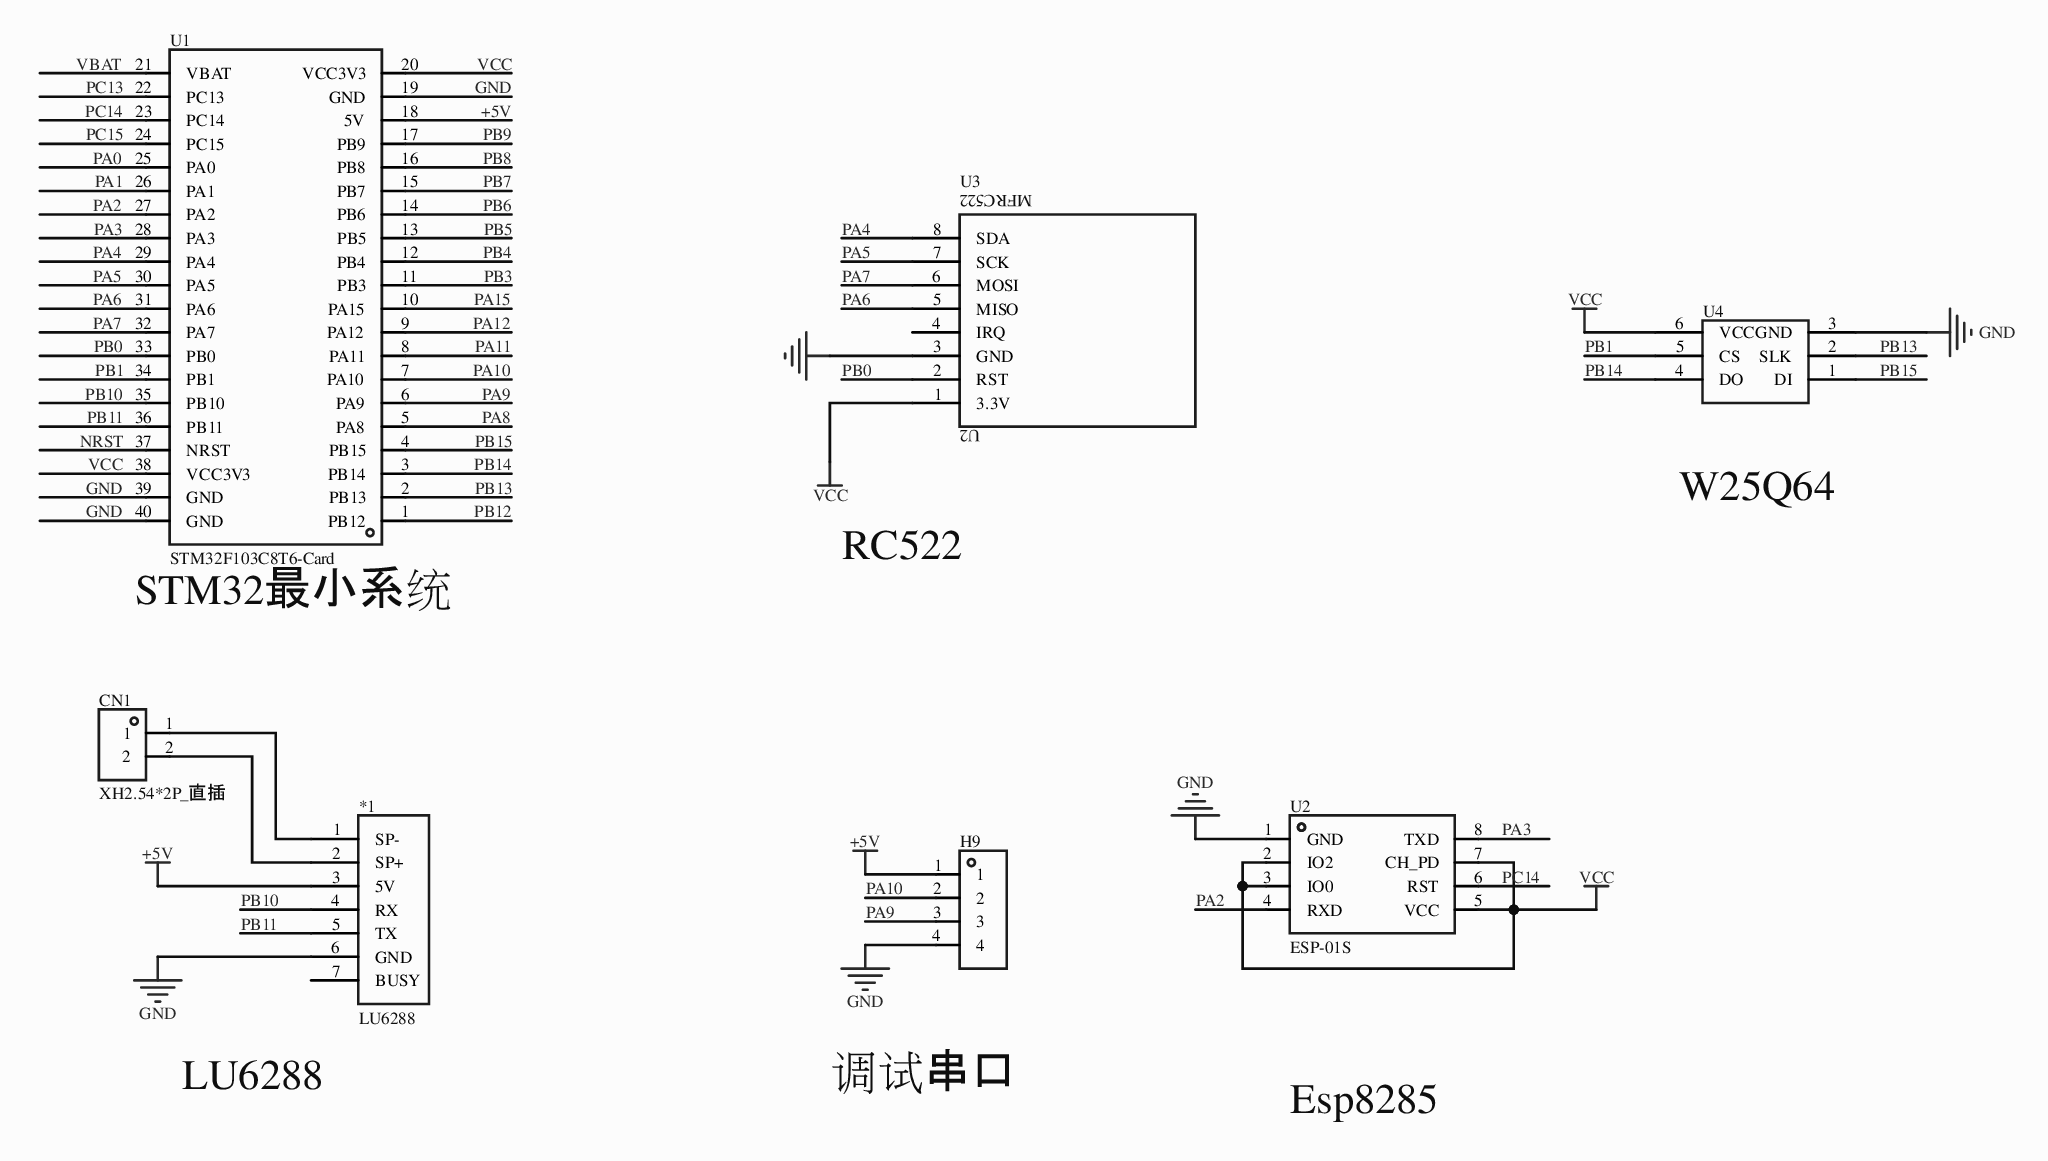
[diagram p0: MISC51107-3.schdoc]
# Altium project MISC51107-2.PrjPcb
1 sheet, 7 parts. Net scope: global (net labels, ports and power ports of the same name join across sheets).
Board file: MISC51107.pcbdoc

## Sheet MISC51107-3.schdoc
size 297 x 209 mm; Version: V1.0; @Project Name: MISC51107; @Page Count: 1; @Update Date: 2026-05-15; @Create Date: 2026-05-15; @Schematic Name: MISC51107; @Page No: 1; @Create Time: 23:22:16; @Update Time: 17:32:40; @Board Name: MISC51107

### Parts
*1  LU6288  [LU6288]
CN1  XH2.54*2P_直插  [CONN-TH_2P-P2.50-XH2.54-2P]
H9  (no value)  [HDR-TH_4P-P2.54-V-M]
U1  STM32F103C8T6-Card  [CONN-TH_L53.3-W22.9_STM32F103C8T6-CARD]
U2  ESP-01S  [WIFIM-TH_ESP-01S]
U3  (no value)  [RC522]
U4  (no value)  [W25Q64]

### Nets
+5V: *1.3(5V) H9.1 U1.18(5V)
GND: *1.6(GND) H9.4 U1.19(GND) U1.39(GND) U1.40(GND) U2.1(GND) U3.3(GND) U4.3(GND)
VCC: U1.20(VCC3V3) U1.38(VCC3V3) U2.2(IO2) U2.3(IO0) U2.5(VCC) U2.7(CH_PD) U3.1(3.3V) U4.6(VCC)
NRST: U1.37(NRST)
PA0: U1.25(PA0)
PA1: U1.26(PA1)
PA2: U1.27(PA2) U2.4(RXD)
PA3: U1.28(PA3) U2.8(TXD)
PA4: U1.29(PA4) U3.8(SDA)
PA5: U1.30(PA5) U3.7(SCK)
PA6: U1.31(PA6) U3.5(MISO)
PA7: U1.32(PA7) U3.6(MOSI)
PA8: U1.5(PA8)
PA9: H9.3 U1.6(PA9)
PA10: H9.2 U1.7(PA10)
PA11: U1.8(PA11)
PA12: U1.9(PA12)
PA15: U1.10(PA15)
PB0: U1.33(PB0) U3.2(RST)
PB1: U1.34(PB1) U4.5(CS)
PB3: U1.11(PB3)
PB4: U1.12(PB4)
PB5: U1.13(PB5)
PB6: U1.14(PB6)
PB7: U1.15(PB7)
PB8: U1.16(PB8)
PB9: U1.17(PB9)
PB10: *1.4(RX) U1.35(PB10)
PB11: *1.5(TX) U1.36(PB11)
PB12: U1.1(PB12)
PB13: U1.2(PB13) U4.2(SLK)
PB14: U1.3(PB14) U4.4(DO)
PB15: U1.4(PB15) U4.1(DI)
PC13: U1.22(PC13)
PC14: U1.23(PC14) U2.6(RST)
PC15: U1.24(PC15)
VBAT: U1.21(VBAT)
Net*1_1: *1.1(SP-) CN1.1
Net*1_2: *1.2(SP+) CN1.2

Not connected (* = marked no-connect by the designer): *1 7(BUSY); U3 4(IRQ)

### Notes on the sheet
- RC522 SPI1
  SDA  PA4
  SCK  PA5
  MISO PA6
  MOSI PA7
  RST PB0
  IRQ 悬空
  VCC 3V3
  GND GND
  W25Q64 SPI2
  CS PB1
  CLK PB13
  DI PB15
  DO PB14
  VCC 3V3
  GND GND
  ESP8285 USART2
  TXD PA3
  RXD PA2
  RST PC14
  EN 3V3
  IO0 3V3
  IO2 3V3
  VCC 3V3
  GND GND
  LU6288 USART3
  RXD PB10
  TXD PB11
  SPK+ 喇叭+
  SPK- 喇叭-
  VCC 3V3
  GND GND
  调试串口USB-T
  TXD PA10
  RXD PA9
  GND GND
  识别模块RC522
- RC522
- (near U4) W25Q64
- (near U1) STM32最小系统
- (near *1) LU6288
- 调试串口
- Esp8285

### Library data of the parts
*1 = LU6288: AddInBom: yes; Symbol: LU6288; Device: LU6288; ConvertToPcb: yes; FootprintName: LU6288
CN1 = XH2.54*2P_直插: AddInBom: yes; ModelId: 325c595e30db4df8abe76612dd40b0fa0819f05c4eef4c71ace90d822a990e87; ModelTransform: 295.275,228.346,0,180,0,0,-0.002,-20.079,-137.795; Symbol: XH2.54*2P_直插; Device: XH2.54*2P_直插; LCSC Part Name: XH2.54*2P_直插; SupplierPart: C9900008615; ManufacturerPart: XH2.54*2P_直插; Supplier Footprint: XH2.54_2P; JLCPCB Part Class: Extended Part; Supplier: LCSC; ConvertToPcb: yes; FootprintName: CONN-TH_2P-P2.50-XH2.54-2P; ModelName: CONN-TH_2P-P2.50-XH2.54-2P
H9 = HDR-M_2.54_1x4P: Symbol: PZ254V-11-04P; ConvertToPcb: yes; ModelId: 112f4d05e8d64e99ab9a333894bea4f90819f05c4eef4c71ace90d822a990e87; ModelName: HDR-TH_4P-P2.54-M-LI-1X4P; ModelTransform: 399.999,104.7242,0,0,0,0,0,0,-118.11; Device: HDR-M_2.54_1x4P; AddInBom: yes; SupplierPart: C492403; Supplier Footprint: 插件; FootprintName: HDR-TH_4P-P2.54-V-M
U1 = STM32F103C8T6-Card: AddInBom: yes; Device: STM32F103C8T6-Card; Symbol: STM32F103C8T6-CARD; FootprintName: CONN-TH_L53.3-W22.9_STM32F103C8T6-CARD; LCSC Part Name: STM32F103C8T6-Card; SupplierPart: C9900077949; ManufacturerPart: STM32F103C8T6-Card; Supplier Footprint: 插件; Supplier: LCSC; ConvertToPcb: yes
U2 = ESP-01S_C111009: AddInBom: yes; ModelId: eb7175da78ae48b3b1568cfe3027405f0819f05c4eef4c71ace90d822a990e87; ModelTransform: 582.676,976.37608,0,0,0,0,0,388.346,-118.11; Symbol: ESP-01S; Device: ESP-01S_C111009; LCSC Part Name: ESP-01S; SupplierPart: C111009; ManufacturerPart: ESP-01S; Supplier Footprint: -; JLCPCB Part Class: Extended Part; Supplier: LCSC; ConvertToPcb: yes; FootprintName: WIFIM-TH_ESP-01S; ModelName: WIFIM-TH_ESP-01S
U3 = RC522: AddInBom: yes; Symbol: RC522; Device: RC522; ConvertToPcb: yes; FootprintName: RC522
U4 = W25Q64: AddInBom: yes; Symbol: W25Q64; Device: W25Q64; ConvertToPcb: yes; FootprintName: W25Q64